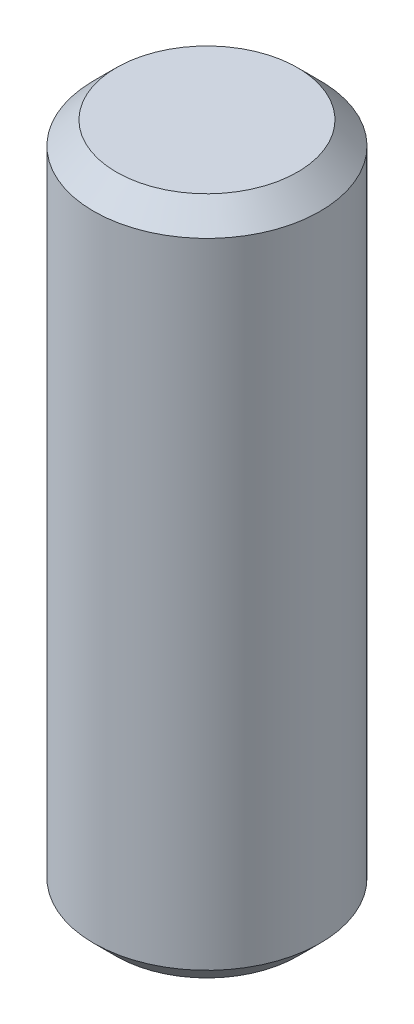
SolidWorks part; units mm, degrees
ref_plane "前视基准面" through (0, 0, 0) normal (0, 0, 1) x (1, 0, 0)
ref_plane "上视基准面" through (0, 0, 0) normal (0, 1, 0) x (1, 0, 0)
ref_plane "右视基准面" through (0, 0, 0) normal (1, 0, 0) x (0, 0, -1)
sketch "草图1" plane through (0, 0, 0) normal (0, 1, 0) x (1, 0, 0)
  circle A0 centre (0, 0) radius 2.5
  dimension "D1" = 5
extrude "凸台-拉伸1" add sketch "草图1" along normal blind 15
hole_wizard "M3 螺纹孔1" positions "草图2" profile "草图3" tap size "M3" standard "GB"
sketch "草图2" plane through (0, 0, 0) normal (0, -1, 0) x (-1, 0, 0)
  point P0 (0, 0)
sketch "草图3" plane through (0, 0, 0) normal (1, 0, 0) x (0, 0, -1)
  line L0 (0, 0) -> (0, 8.2511)
  line L1 (0, 8.2511) -> (1.25, 7.5)
  line L2 (1.25, 7.5) -> (1.25, 0)
  line L5 (1.25, 0) -> (0, 0)
  line L10 (0, 8.2511) -> (-1.25, 7.5) construction
  line L11 (0, -6.35) -> (0, 107.95) construction
  dimension "螺纹孔钻头直径" = 2.5
  dimension "螺纹孔钻头深度" = 7.5
  dimension "导头角度" = 118
cosmetic thread "孔螺蚊线1" parameters "D1"=6, "D2"=3
chamfer "倒角1" distance 0.5 angle 45 2 edges at (0, 0, 2.5) (0, 15, 2.5)
